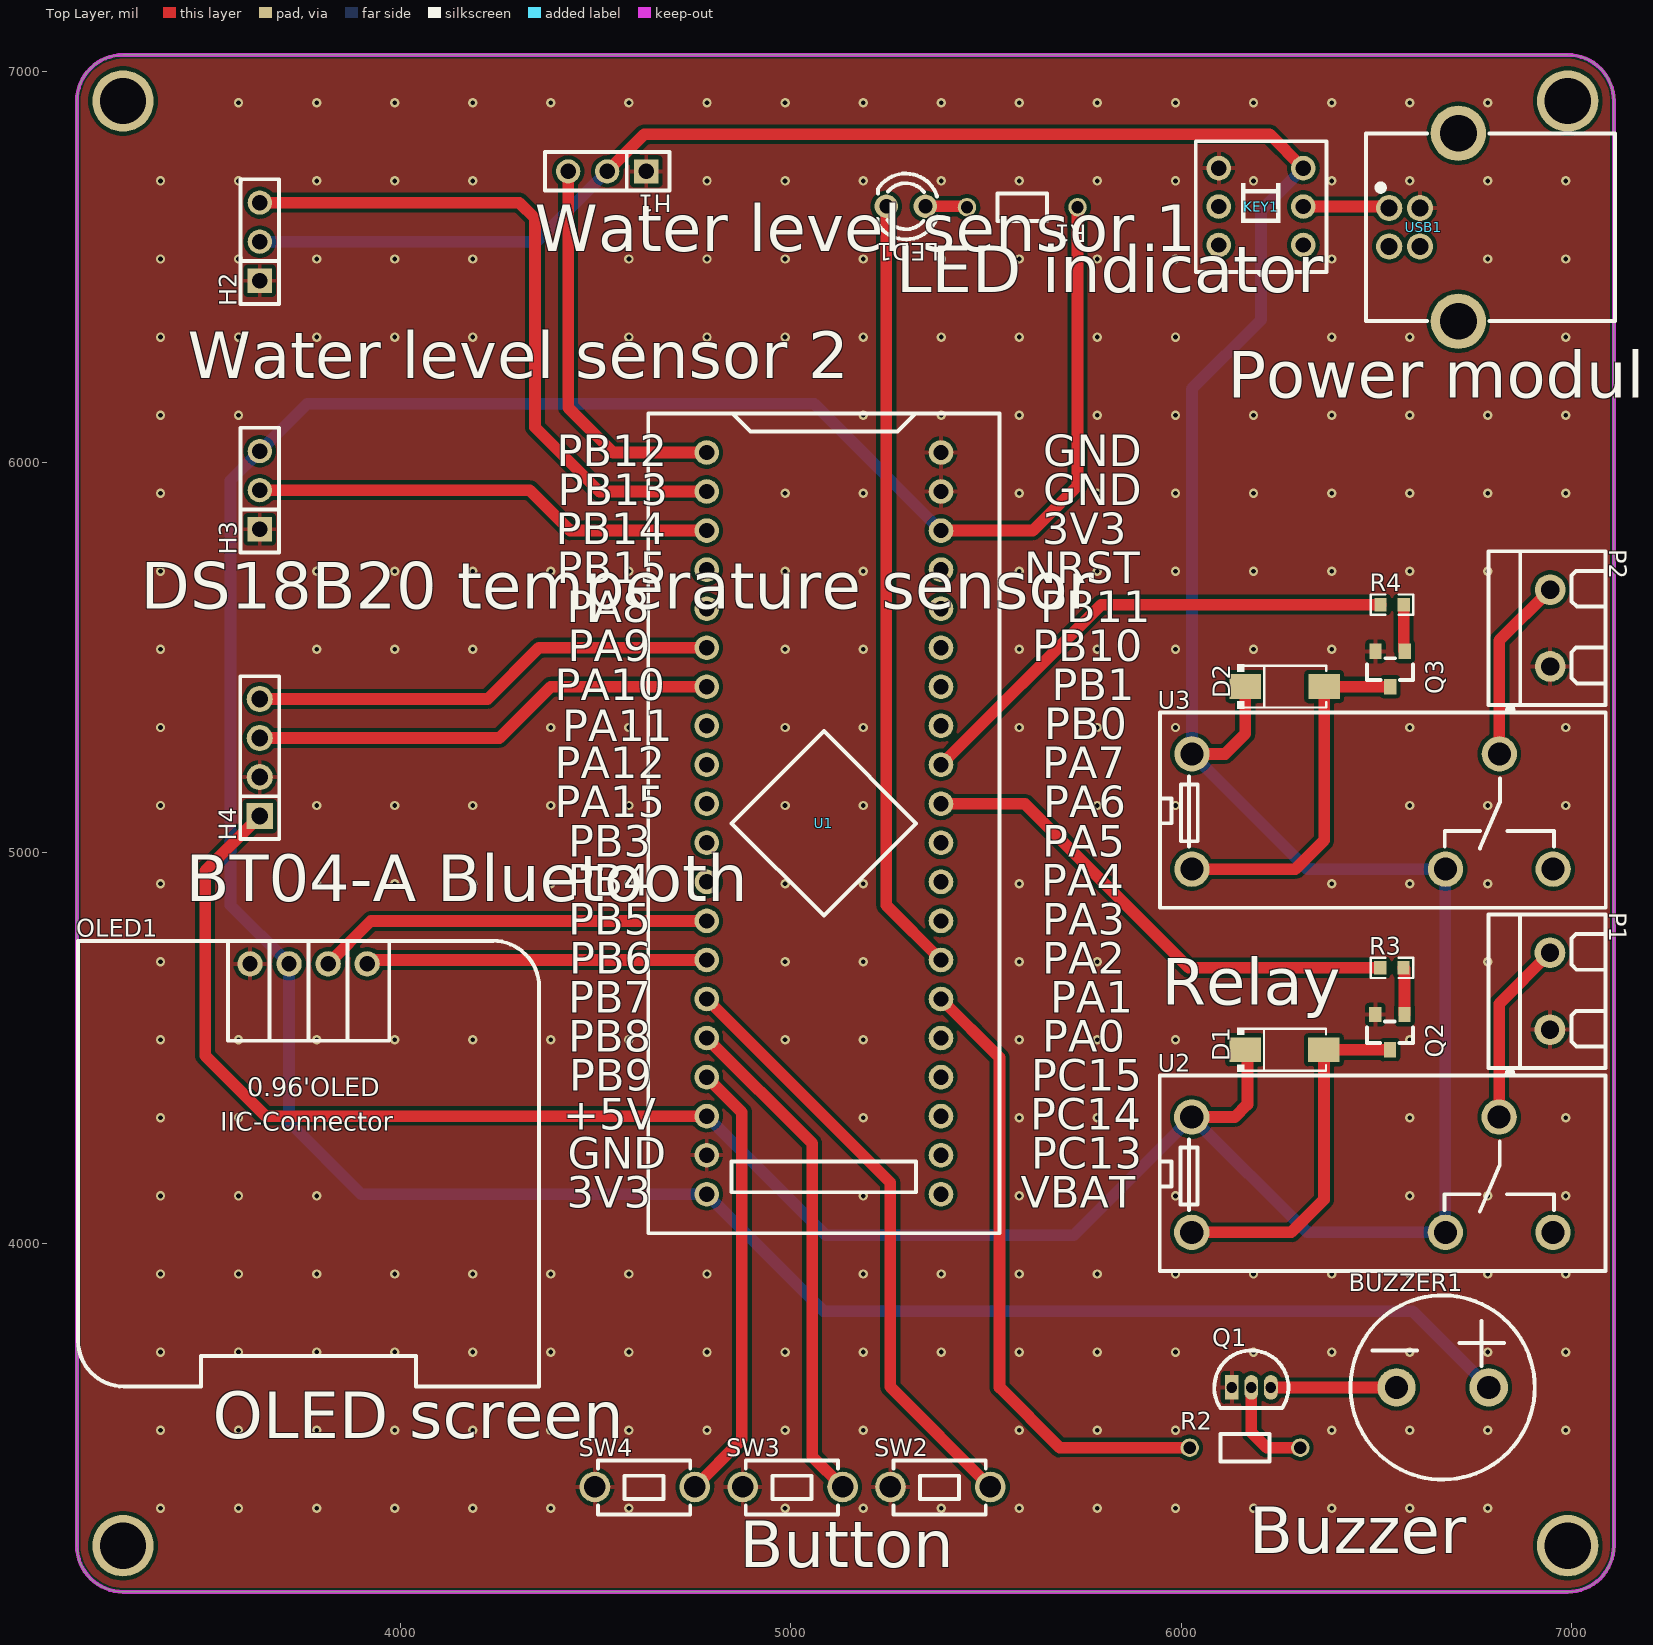
[diagram p0: Top Layer view]
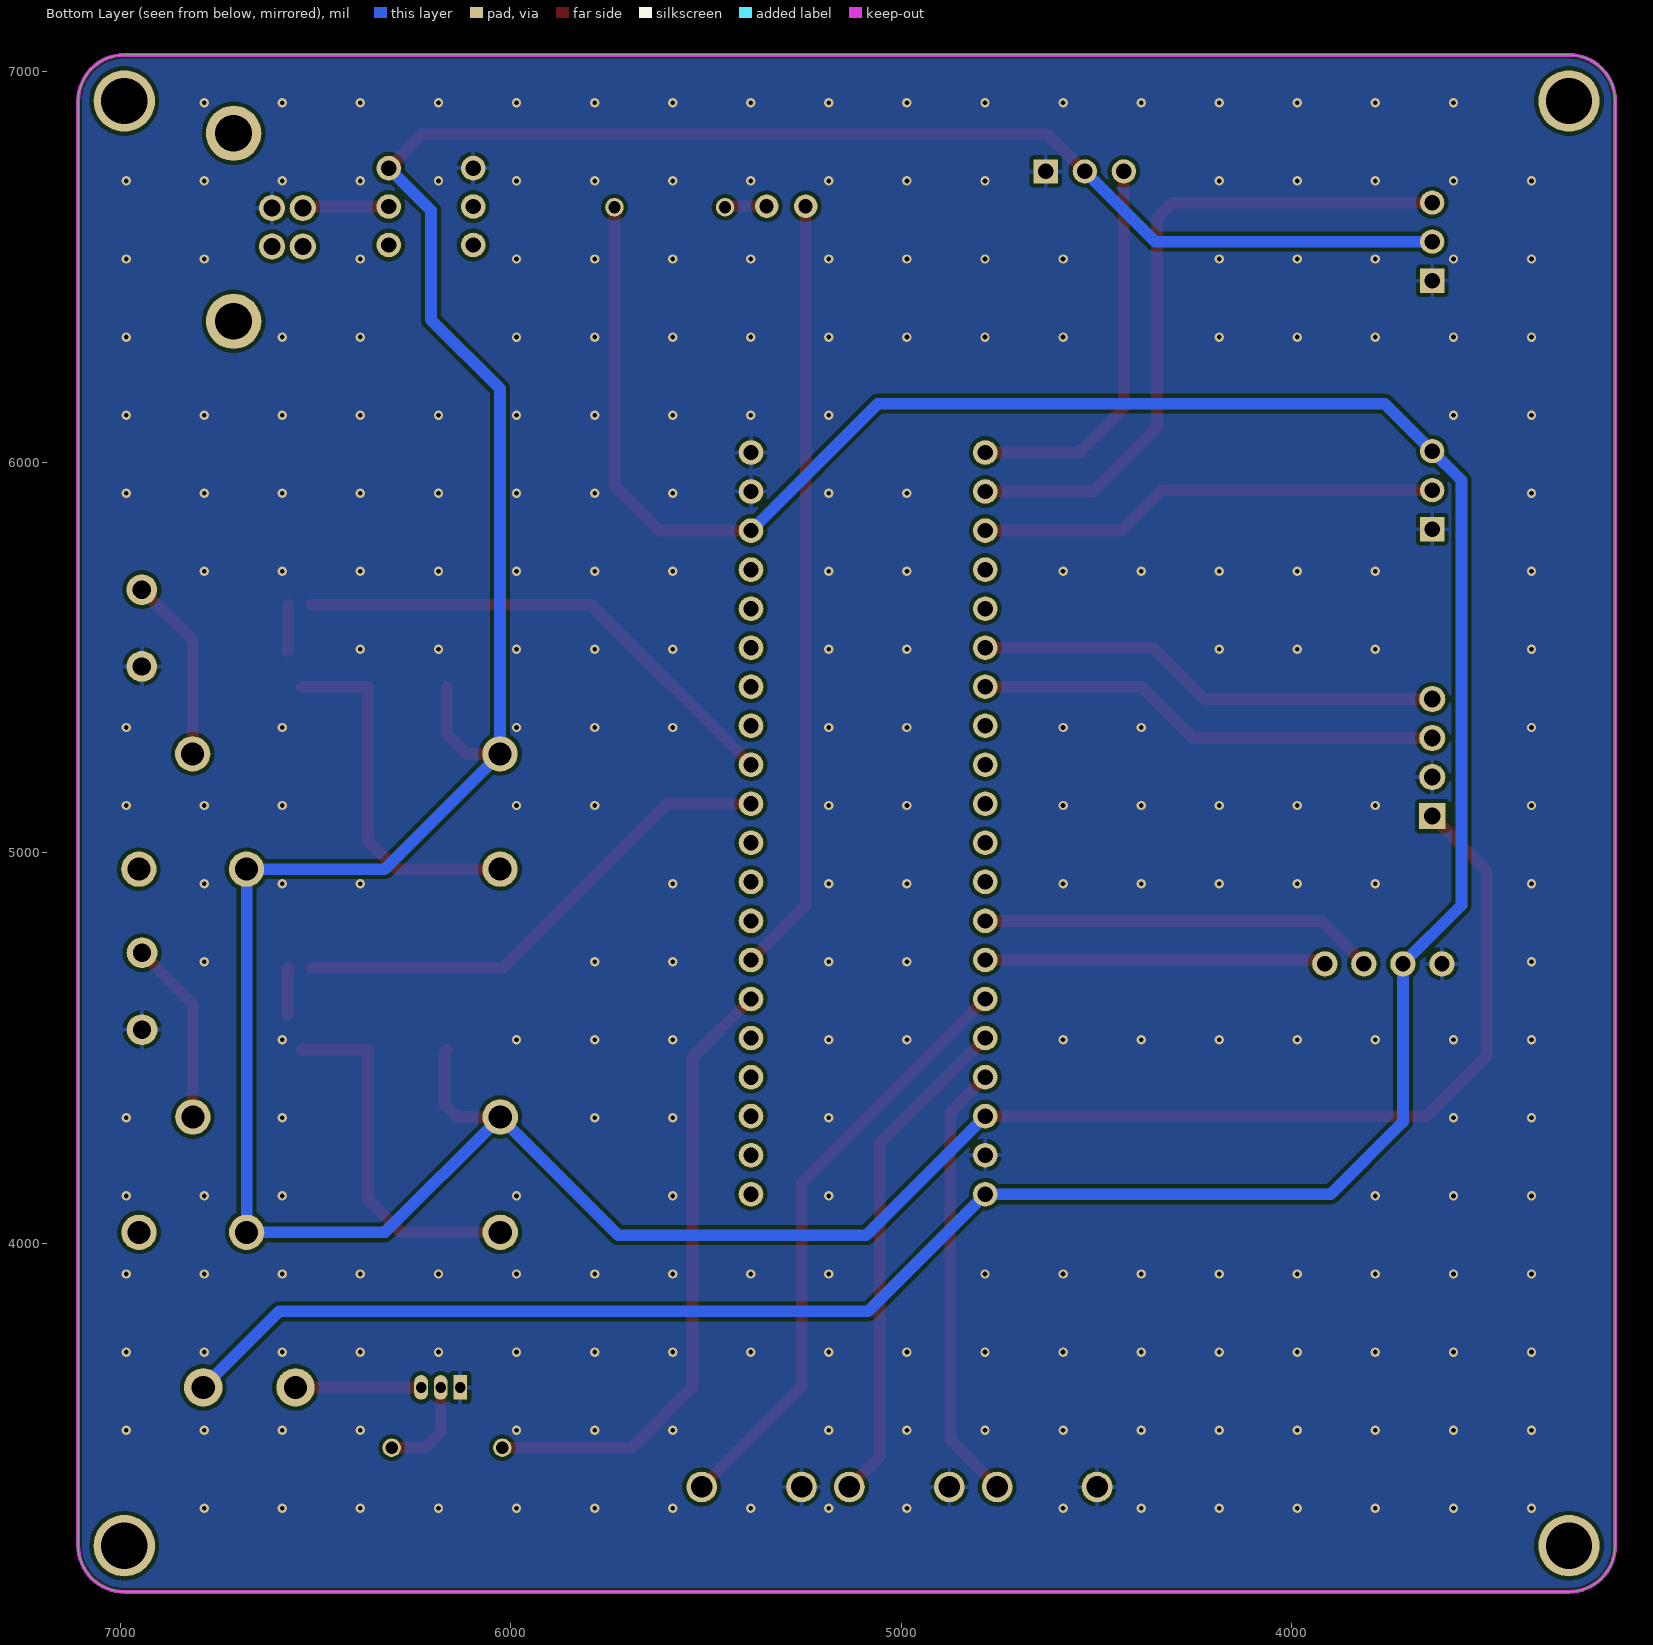
[diagram p1: Bottom Layer view, seen from below]
# Altium PCB MISC89014.pcbdoc
Units mil, origin at the board's own origin, x right, y up, seen from the top; angles counter-clockwise.
Board outline 3937.01 x 3937.01 mil, 2 copper layers (Top Layer, Bottom Layer), stack 62.206 mil thick; 26 components, 47 nets, 118 pads, 256 vias.

## Layer stack, top to bottom
Top Solder Mask Layer: solder mask 0.394, Dk 3.3
Top Layer: signal copper 1.379
Dielectric1: surface 59.449, FR4, Dk 4.5
Bottom Layer: signal copper 1.378
Bottom Solder Mask Layer: solder mask 0.394, Dk 3.3

## Board outline
6990.39,3106.5 ccw(c6990.39,3224.61) 7108.5,3224.61 7108.5,6925.39 ccw(c6990.39,6925.39) 6990.39,7043.5 3289.61,7043.5 ccw(c3289.61,6925.39) 3171.5,6925.39 3171.5,3224.61 ccw(c3289.61,3224.61) 3289.61,3106.5

## Design rules (kind name [scope] priority, off if disabled: settings)
BoardOutlineClearance copperThickness2oz_1 [All] p2 off: genericclearance=7.99 ignorepadtopadclearanceinfootprint=FALSE except(0: Arc-SplitContinuation Track-SplitContinuation SMDPad-SplitContinuation THPad-SplitContinuation Via-SplitContinuation Fill-SplitContinuation Region-SplitContinuation Poly-SplitContinuation Text-SplitContinuation Hole-SplitContinuation; 5.98: Arc-CutoutEdge Track-CutoutEdge SMDPad-CutoutEdge THPad-CutoutEdge Via-CutoutEdge Text-CutoutEdge; 6.89: Hole-OutlineEdge Hole-CutoutEdge; 10: Poly-OutlineEdge Poly-CutoutEdge; 11.81: Arc-OutlineEdge Track-OutlineEdge SMDPad-OutlineEdge THPad-OutlineEdge Via-OutlineEdge Fill-OutlineEdge Region-OutlineEdge Text-OutlineEdge Fill-CutoutEdge Region-CutoutEdge)
BoardOutlineClearance Plane_innerPlane_1 [All] p4 off: genericclearance=4.02 ignorepadtopadclearanceinfootprint=FALSE except(0: Arc-SplitContinuation Track-SplitContinuation SMDPad-SplitContinuation THPad-SplitContinuation Via-SplitContinuation Fill-SplitContinuation Region-SplitContinuation Poly-SplitContinuation Text-SplitContinuation Hole-SplitContinuation; 5.98: Arc-CutoutEdge Track-CutoutEdge SMDPad-CutoutEdge THPad-CutoutEdge Via-CutoutEdge Text-CutoutEdge; 6.89: Hole-OutlineEdge Hole-CutoutEdge; 10: Poly-OutlineEdge Poly-CutoutEdge; 11.81: Arc-OutlineEdge Track-OutlineEdge SMDPad-OutlineEdge THPad-OutlineEdge Via-OutlineEdge Fill-OutlineEdge Region-OutlineEdge Text-OutlineEdge Fill-CutoutEdge Region-CutoutEdge)
BoardOutlineClearance Copper_copperRegion_1 [All] p6 off: genericclearance=4.02 ignorepadtopadclearanceinfootprint=FALSE except(0: Arc-SplitContinuation Track-SplitContinuation SMDPad-SplitContinuation THPad-SplitContinuation Via-SplitContinuation Fill-SplitContinuation Region-SplitContinuation Poly-SplitContinuation Text-SplitContinuation Hole-SplitContinuation; 5.98: Arc-CutoutEdge Track-CutoutEdge SMDPad-CutoutEdge THPad-CutoutEdge Via-CutoutEdge Text-CutoutEdge; 6.89: Hole-OutlineEdge Hole-CutoutEdge; 10: Poly-OutlineEdge Poly-CutoutEdge; 11.81: Arc-OutlineEdge Track-OutlineEdge SMDPad-OutlineEdge THPad-OutlineEdge Via-OutlineEdge Fill-OutlineEdge Region-OutlineEdge Text-OutlineEdge Fill-CutoutEdge Region-CutoutEdge)
BoardOutlineClearance copperThickness1oz_1 [All] p8: genericclearance=4.02 ignorepadtopadclearanceinfootprint=FALSE except(0: Arc-SplitContinuation Track-SplitContinuation SMDPad-SplitContinuation THPad-SplitContinuation Via-SplitContinuation Fill-SplitContinuation Region-SplitContinuation Poly-SplitContinuation Text-SplitContinuation Hole-SplitContinuation; 5.98: Arc-CutoutEdge Track-CutoutEdge SMDPad-CutoutEdge THPad-CutoutEdge Via-CutoutEdge Text-CutoutEdge; 6.89: Hole-OutlineEdge Hole-CutoutEdge; 10: Poly-OutlineEdge Poly-CutoutEdge; 11.81: Arc-OutlineEdge Track-OutlineEdge SMDPad-OutlineEdge THPad-OutlineEdge Via-OutlineEdge Fill-OutlineEdge Region-OutlineEdge Text-OutlineEdge Fill-CutoutEdge Region-CutoutEdge)
Clearance copperThickness2oz [All] p1 off: gap=7.99 ignorepadtopadclearanceinfootprint=FALSE except(5.98: SMDPad-Track SMDPad-SMDPad THPad-Track SMDPad-THPad THPad-THPad Track-Via SMDPad-Via THPad-Via Via-Via Fill-SMDPad Region-SMDPad Fill-THPad Region-THPad Fill-Via Region-Via Fill-Fill Fill-Region Region-Region Arc-Track Arc-SMDPad Arc-THPad Arc-Via Fill-Arc Region-Arc Arc-Arc Text-Track SMDPad-Text Text-THPad Text-Via Fill-Text Region-Text Arc-Text Text-Text; 6.89: Hole-Track Hole-SMDPad Hole-THPad Hole-Via Fill-Hole Region-Hole Hole-Arc Hole-Text; 10: Poly-Track Poly-SMDPad Poly-THPad Poly-Via Poly-Fill Poly-Region Poly-Poly Poly-Arc Poly-Text Poly-Hole; 11.81: Fill-Track Region-Track)
Clearance Plane_innerPlane [All] p3 off: gap=4.02 ignorepadtopadclearanceinfootprint=FALSE except(5.98: SMDPad-Track SMDPad-SMDPad THPad-Track SMDPad-THPad THPad-THPad Track-Via SMDPad-Via THPad-Via Via-Via Fill-SMDPad Region-SMDPad Fill-THPad Region-THPad Fill-Via Region-Via Fill-Fill Fill-Region Region-Region Arc-Track Arc-SMDPad Arc-THPad Arc-Via Fill-Arc Region-Arc Arc-Arc Text-Track SMDPad-Text Text-THPad Text-Via Fill-Text Region-Text Arc-Text Text-Text; 6.89: Hole-Track Hole-SMDPad Hole-THPad Hole-Via Fill-Hole Region-Hole Hole-Arc Hole-Text; 10: Poly-Track Poly-SMDPad Poly-THPad Poly-Via Poly-Fill Poly-Region Poly-Poly Poly-Arc Poly-Text Poly-Hole; 11.81: Fill-Track Region-Track)
Clearance Copper_copperRegion [All] p5 off: gap=4.02 ignorepadtopadclearanceinfootprint=FALSE except(5.98: SMDPad-Track SMDPad-SMDPad THPad-Track SMDPad-THPad THPad-THPad Track-Via SMDPad-Via THPad-Via Via-Via Fill-SMDPad Region-SMDPad Fill-THPad Region-THPad Fill-Via Region-Via Fill-Fill Fill-Region Region-Region Arc-Track Arc-SMDPad Arc-THPad Arc-Via Fill-Arc Region-Arc Arc-Arc Text-Track SMDPad-Text Text-THPad Text-Via Fill-Text Region-Text Arc-Text Text-Text; 6.89: Hole-Track Hole-SMDPad Hole-THPad Hole-Via Fill-Hole Region-Hole Hole-Arc Hole-Text; 10: Poly-Track Poly-SMDPad Poly-THPad Poly-Via Poly-Fill Poly-Region Poly-Poly Poly-Arc Poly-Text Poly-Hole; 11.81: Fill-Track Region-Track)
Clearance copperThickness1oz [All] p7: gap=4.02 ignorepadtopadclearanceinfootprint=FALSE except(5.98: SMDPad-Track SMDPad-SMDPad THPad-Track SMDPad-THPad THPad-THPad Track-Via SMDPad-Via THPad-Via Via-Via Fill-SMDPad Region-SMDPad Fill-THPad Region-THPad Fill-Via Region-Via Fill-Fill Fill-Region Region-Region Arc-Track Arc-SMDPad Arc-THPad Arc-Via Fill-Arc Region-Arc Arc-Arc Text-Track SMDPad-Text Text-THPad Text-Via Fill-Text Region-Text Arc-Text Text-Text; 6.89: Hole-Track Hole-SMDPad Hole-THPad Hole-Via Fill-Hole Region-Hole Hole-Arc Hole-Text; 10: Poly-Track Poly-SMDPad Poly-THPad Poly-Via Poly-Fill Poly-Region Poly-Poly Poly-Arc Poly-Text Poly-Hole; 11.81: Fill-Track Region-Track)
DiffPairsRouting differentialPair [All] p1: maxlimit=6 minlimit=6 mostfreqgap=6 toplayer_minwidth=5 toplayer_prefwidth=10 toplayer_maxwidth=100 toplayer_mingap=6 toplayer_prefgap=6 toplayer_maxgap=6 bottomlayer_minwidth=5 bottomlayer_prefwidth=10 bottomlayer_maxwidth=100 bottomlayer_mingap=6 bottomlayer_prefgap=6 bottomlayer_maxgap=6 maxuncoupledlength=10
HoleToHoleClearance otherClearance [All] p1: gap=11.81 allowstackedmicrovias=TRUE
Length netLength [All] p1: minlimit=0 maxlimit=0
PasteMaskExpansion pasteMaskExpansion [All] p1: expansion=0
PlaneConnect innerPlane [All] p1: planeconnectstyle=Relief reliefexpansion=20 reliefentries=4 reliefconductorwidth=10 reliefairgap=10
PolygonConnect copperRegion [All] p1: connectstyle=Relief reliefconductorwidth=10 reliefentries=4 polygonreliefangle="90 Angle" airgapwidth=10 via.connectstyle=Relief via.reliefconductorwidth=10 via.reliefentries=4 via.polygonreliefangle="90 Angle" via.airgapwidth=10
RoutingVias viaSize [All] p1: holewidth=12.01 width=24.02 viastyle="Through Hole" minholewidth=11.81 minwidth=19.68 maxholewidth=248.03 maxwidth=393.7
SolderMaskExpansion solderMaskExpansion [IsVia] p1: expansion=-1000 istentingtop=TRUE
SolderMaskExpansion solderMaskExpansion [All] p2: expansion=2.01 istentingtop=FALSE
Width copperThickness2oz_2 [All] p1 off: maxlimit=100 minlimit=8 preferedwidth=10
Width copperThickness1oz_2 [All] p2: maxlimit=100 minlimit=5 preferedwidth=30

## Components (designator, comment, footprint, x,y, rotation, side; value= is the part's Value field where it differs from the comment)
BUZZER1 "buzzer" BUZ-TH_BD12.0-P6.00-D0.9-RD 6670,3630 r0 top
D1 "" SMA_1N4007 6265,4495 r0 top
D2 "" SMA_1N4007 6265.47,5425.24 r0 top
H1 "" HDR-TH_3P-P2.54-V-F 4530,6745 r180 top
H2 "" HDR-TH_3P-P2.54-V-F 3640,6565 r90 top
H3 "" HDR-TH_3P-P2.54-V-F 3640,5928.44 r90 top
H4 "" HDR-TH_4P-P2.54-V-F 3640,5243.46 r90 top
KEY1 "Non-self-locking switch 8.5×8.5 silent" SW-TH_6P-L8.5-W8.5-P2.54 6205,6655 r90 top
LED1 "" LED_TH-3mm 5294.9,6655.74 r180 top
OLED1 "" 0.96OLED_4P 3765,4715 r0 top
P1 "KF301-2P terminal block" CONN-TH_XY301V-A-5.0-2P 6945,4645 r270 top
P2 "KF301-2P terminal block" CONN-TH_XY301V-A-5.0-2P 6945.47,5575.24 r270 top
Q1 "" S8050_TO_92 6180,3630 r0 top
Q2 "" S8050_SOT-23 6535,4540 r90 top
Q3 "" S8050_SOT-23 6535.47,5470.24 r90 top
R1 "220" Res_1/8W 5593.23,6655.74 r180 top
R2 "10kΩ" Res_1/8W 6163.81,3473.19 r0 top
R3 "1K" R0603 6540,4705 r0 top
R4 "1K" R0603 6540.47,5635.24 r0 top
SW2 "" Key_TH_3.5x6x4.3 5377.07,3375 r0 top
SW3 "" Key_TH_3.5x6x4.3 4998.53,3375 r0 top
SW4 "" Key_TH_3.5x6x4.3 4620,3375 r0 top
U1 "STM32F103C8T6-Card" CONN-TH_L53.3-W22.9_STM32F103C8T6-CARD 5085,5075 r270 top
U2 "SSKD6132" RELAY-TH_G2R-1 6490,4175 r0 top
U3 "SSKD6132" RELAY-TH_G2R-1 6490.47,5105.24 r0 top
USB1 "" "USB_ Type-B" 6790.29,6596.4 r90 top

## Footprints (in the part's own frame and the unit in brackets; to place one, negate y for a bottom-side part, rotate by r counter-clockwise, add the part's x,y. Pads: shape width x height; smd on the part's side, far side on the other; paste and mask are expansions set on the pad)
0.96OLED_4P [mm]
  round 1.65 hole 1 copper offset 0,0: 1(-3.81,-0.001) 2(-1.27,0.002) 3(1.27,0.002) 4(3.81,0.002)
  silkscreen extent -15,-27.5 15,1.5
BUZ-TH_BD12.0-P6.00-D0.9-RD [mm]
  round 2.5 hole 1.5 paste+0 mask+0.05: 1(-3,0) 2(3,0)
  silkscreen extent -5.99,-5.99 5.99,5.99
CONN-TH_L53.3-W22.9_STM32F103C8T6-CARD [mm]
  round 1.6 hole 1: 1(-24.13,-7.62) 2(-21.59,-7.62) 3(-19.05,-7.62) 4(-16.51,-7.62) 5(-13.97,-7.62) 6(-11.43,-7.62) 7(-8.89,-7.62) 8(-6.35,-7.62) 9(-3.81,-7.62) 10(-1.27,-7.62) 11(1.27,-7.62) 12(3.81,-7.62) 13(6.35,-7.62) 14(8.89,-7.62) 15(11.43,-7.62) 16(13.97,-7.62) 17(16.51,-7.62) 18(19.05,-7.62) 19(21.59,-7.62) 20(24.13,-7.62) 21(24.13,7.62) 22(21.59,7.62) 23(19.05,7.62) 24(16.51,7.62) 25(13.97,7.62) 26(11.43,7.62) 27(8.89,7.62) 28(6.35,7.62) 29(3.81,7.62) 30(1.27,7.62) 31(-1.27,7.62) 32(-3.81,7.62) 33(-6.35,7.62) 34(-8.89,7.62) 35(-11.43,7.62) 36(-13.97,7.62) 37(-16.51,7.62) 38(-19.05,7.62) 39(-21.59,7.62) 40(-24.13,7.62)
  silkscreen extent -26.67,-11.43 26.67,11.43
CONN-TH_XY301V-A-5.0-2P [mm]
  round 2 hole 1.2: 1(-2.5,0) 2(2.5,0)
  silkscreen extent -5,-4 5.6,3.6
HDR-TH_3P-P2.54-V-F [mil]
  rect 62x62 hole 40.16: 1(-100,0)
  round 62 hole 40.16: 2(0,0) 3(100,0)
  silkscreen extent -160,-49 160,49
HDR-TH_4P-P2.54-V-F [mm]
  rect 1.7x1.7 hole 1.1: 1(-3.81,0)
  round 1.7 hole 1.1: 2(-1.27,0) 3(1.27,0) 4(3.81,0)
  silkscreen extent -5.29,-1.27 5.29,1.27
Key_TH_3.5x6x4.3 [mil]
  round 78.7 hole 55.1 paste+0 mask+2: A(-121.44,0) B(134.46,0)
  silkscreen extent -114,-70 123,68
LED_TH-3mm [mil]
  round 60 hole 36 paste+0 mask+2: 1(-50,0) 2(50,0)
  silkscreen extent -81,-84 72,85
R0603 [mil]
  rect 31.75x34.02 smd paste-3937.01 mask+2: 1(-29.66,0) 2(29.66,0)
  silkscreen extent -55,-26 55,26
RELAY-TH_G2R-1 [mm]
  round 2.3 hole 1.5: 1(-11.75,-3.75) 2(4.75,-3.75) 3(11.75,-3.75) 4(8.25,3.75) 5(-11.75,3.75)
  silkscreen extent -13.83,-6.26 15.17,6.44
Res_1/8W [mil]
  round 47.2 hole 31.5 paste+0 mask+2: 1(-141.7,2.48) 2(141.7,2.48)
  silkscreen extent -63,-33 63,38
S8050_SOT-23 [mm]
  rect 1x0.8 smd paste+0 mask+0.051: 1(1.15,-0.95) 2(1.15,0.95) 3(-1.15,0)
  silkscreen extent -0.7,-1.5 0.7,1.5
S8050_TO_92 [mil]
  rect 35.4x63 hole 27.6 paste+0 mask+2: 1(-50,0)
  oval 35.4x63 hole 27.6 paste+0 mask+2: 2(0,0) 3(50,0)
  silkscreen extent -95,-53 95,95
SMA_1N4007 [mil]
  rect 80.57x63.78 smd paste+0 mask+2: 1(-101,0) 2(101,0)
  silkscreen extent -121,-57 106,57
SW-TH_6P-L8.5-W8.5-P2.54 [mm]
  round 1.6 hole 1: 1(-2.5,-2.75) 2(0,-2.75) 3(2.5,-2.75) 4(-2.5,2.75) 5(0,2.75) 6(2.5,2.75)
  silkscreen extent -4.47,-4.25 4.25,4.25
"USB_ Type-B" [mm]
  round 1.7 hole 1.1 copper offset 0,0 paste+0 mask+0.051: 1(1.39,6.532) 2(-1.11,6.532) 3(-1.11,4.532) 4(1.39,4.532)
  round 3.6 hole 2.4 paste+0 mask+0.051: 5(-5.977,2.032) 5(6.256,2.032)
  silkscreen extent -5.96,-8.17 6.25,8.03

## Free pads (board coordinates)
  round 157.48 hole 118.11: 1(3289.61,6925.39) 1(3289.61,3224.61) 1(6990.39,6925.39) 1(6990.39,3224.61)

## Via types
v1: diameter 24.02, hole 12, Top Layer to Bottom Layer, 256 vias

## Nets (pads, with @x,y where several pads share a name; then routed paths per layer and width w, separated by ;. In a path a pad name is that pad's centre, name@x,y a point inside that pad or via, vN(x,y) a via of type N, cw(c..) or ccw(c..) an arc to the next point about the centre after c; other vN are vias at no path point)
$1N18282: KEY1.2 USB1.1 | length 221.5
  Top Layer w30: KEY1.2 6529.25,6654.99 USB1.1
$1N18294: LED1.1 R1.2 | length 107.7
  Top Layer w30: LED1.1 5449.05,6655.74 R1.2
$1N18316: BUZZER1.1 Q1.3 | length 321.9
  Top Layer w30: Q1.3 BUZZER1.1
$1N18319: Q1.2 R2.2 | length 256.8
  Top Layer w30: Q1.2 6180,3515 6219.34,3475.66 R2.2
$1N18331: D1.2 Q2.3 U2.1 | length 926.4
  Top Layer w30: U2.1 6282.35,4027.35 6366,4111 D1.2 6534.72,4495 Q2.3
$1N18332: Q2.1 R3.2 | length 120.9
  Top Layer w30: R3.2 6572.4,4702.26 Q2.1
$1N18336: P1.1 U2.4 | length 474.7
  Top Layer w30: U2.4 6814.8,4613.23 P1.1
$1N18339: P2.1 U3.4 | length 474.7
  Top Layer w30: U3.4 6815.27,5543.47 P2.1
$1N18343: Q3.1 R4.2 | length 120.9
  Top Layer w30: R4.2 6570.13,5518.26 Q3.1
$1N18344: D2.2 Q3.3 U3.1 | length 932.1
  Top Layer w30: U3.1 6292.59,4957.59 6366.47,5031.47 D2.2 6535.19,5425.24 Q3.3
+5V: D1.1 D2.1 H1.2 H2.2 H4.1 KEY1.3 U1.18 U2.2 U2.5 U3.2 U3.5 | length 11008
  Top Layer w30: H4.1 3500,4953.46 3500,4480 3655,4325 U1.18 ; H1.2 4625,6840 6226.69,6840 KEY1.3 ; U2.5 6137.65,4322.65 6170,4355 6170,4489 D1.1 ; U3.5 6112.89,5252.89 6164.47,5304.47 D2.1
  Bottom Layer w30: H2.2 4350,6565 H1.2 ; U1.18 5090,4020 5724.75,4020 U2.5 6322.7,4027.35 U2.2 6677,4957.12 U3.2 6323.17,4957.59 U3.5 6027.87,6187.87 6205,6365 6205,6645.15 KEY1.3
GND: H1.1 H2.1 H3.1 H4.2 KEY1.6 OLED1.1 P1.2 P2.2 Q1.1 Q2.2 Q3.2 SW2.A SW3.A SW4.A U1.19 U1.39 U1.40 USB1.4
  other v1: 3385.6,3320.6 3585.6,3320.6 3785.6,3320.6 3985.6,3320.6 4185.6,3320.6 4385.6,3320.6 4585.6,3320.6 4985.6,3320.6 5185.6,3320.6 5385.6,3320.6 5585.6,3320.6 5785.6,3320.6 5985.6,3320.6 6185.6,3320.6 6385.6,3320.6 6585.6,3320.6 6785.6,3320.6 3385.6,3520.6 3585.6,3520.6 3785.6,3520.6 3985.6,3520.6 4185.6,3520.6 4385.6,3520.6 4585.6,3520.6 4785.6,3520.6 4985.6,3520.6 5185.6,3520.6 5585.6,3520.6 5785.6,3520.6 5985.6,3520.6 6385.6,3520.6 6585.6,3520.6 6785.6,3520.6 6985.6,3520.6 3385.6,3720.6 3585.6,3720.6 3785.6,3720.6 3985.6,3720.6 4185.6,3720.6 4385.6,3720.6 4585.6,3720.6 4785.6,3720.6 4985.6,3720.6 5185.6,3720.6 5385.6,3720.6 5585.6,3720.6 5785.6,3720.6 5985.6,3720.6 6185.6,3720.6 6385.6,3720.6 6585.6,3720.6 6785.6,3720.6 6985.6,3720.6 3385.6,3920.6 3585.6,3920.6 3785.6,3920.6 3985.6,3920.6 4185.6,3920.6 4385.6,3920.6 4585.6,3920.6 4785.6,3920.6 5185.6,3920.6 5385.6,3920.6 5585.6,3920.6 5785.6,3920.6 5985.6,3920.6 6185.6,3920.6 6385.6,3920.6 6585.6,3920.6 6785.6,3920.6 6985.6,3920.6 3385.6,4120.6 3585.6,4120.6 3785.6,4120.6 5185.6,4120.6 5585.6,4120.6 5985.6,4120.6 6585.6,4120.6 6785.6,4120.6 6985.6,4120.6 3385.6,4320.6 3585.6,4320.6 5185.6,4320.6 5585.6,4320.6 5785.6,4320.6 6585.6,4320.6 6985.6,4320.6 3385.6,4520.6 3585.6,4520.6 3785.6,4520.6 3985.6,4520.6 4185.6,4520.6 4385.6,4520.6 4585.6,4520.6 4985.6,4520.6 5185.6,4520.6 5585.6,4520.6 5785.6,4520.6 5985.6,4520.6 6585.6,4520.6 3385.6,4720.6 4985.6,4720.6 5185.6,4720.6 5585.6,4720.6 5785.6,4720.6 6785.6,4720.6 3385.6,4920.6 3785.6,4920.6 3985.6,4920.6 4185.6,4920.6 4385.6,4920.6 4585.6,4920.6 4985.6,4920.6 5185.6,4920.6 5585.6,4920.6 6385.6,4920.6 6585.6,4920.6 6785.6,4920.6 3385.6,5120.6 3785.6,5120.6 3985.6,5120.6 4185.6,5120.6 4385.6,5120.6 4585.6,5120.6 4985.6,5120.6 5185.6,5120.6 5785.6,5120.6 5985.6,5120.6 6585.6,5120.6 6785.6,5120.6 6985.6,5120.6 3385.6,5320.6 4385.6,5320.6 4585.6,5320.6 4985.6,5320.6 5185.6,5320.6 5585.6,5320.6 5785.6,5320.6 5985.6,5320.6 6585.6,5320.6 6985.6,5320.6 3385.6,5520.6 3785.6,5520.6 3985.6,5520.6 4185.6,5520.6 4985.6,5520.6 5185.6,5520.6 5585.6,5520.6 5785.6,5520.6 5985.6,5520.6 6185.6,5520.6 6385.6,5520.6 3385.6,5720.6 3785.6,5720.6 3985.6,5720.6 4185.6,5720.6 4385.6,5720.6 4585.6,5720.6 4985.6,5720.6 5185.6,5720.6 5585.6,5720.6 5785.6,5720.6 5985.6,5720.6 6185.6,5720.6 6385.6,5720.6 6585.6,5720.6 6785.6,5720.6 3385.6,5920.6 4985.6,5920.6 5185.6,5920.6 5585.6,5920.6 5785.6,5920.6 5985.6,5920.6 6185.6,5920.6 6385.6,5920.6 6585.6,5920.6 6785.6,5920.6 6985.6,5920.6 3385.6,6120.6 3585.6,6120.6 5185.6,6120.6 5385.6,6120.6 5585.6,6120.6 5785.6,6120.6 5985.6,6120.6 6185.6,6120.6 6385.6,6120.6 6585.6,6120.6 6785.6,6120.6 6985.6,6120.6 3385.6,6320.6 3585.6,6320.6 3785.6,6320.6 3985.6,6320.6 4185.6,6320.6 4585.6,6320.6 4785.6,6320.6 4985.6,6320.6 5185.6,6320.6 5385.6,6320.6 5585.6,6320.6 5785.6,6320.6 5985.6,6320.6 6385.6,6320.6 6585.6,6320.6 6985.6,6320.6 3385.6,6520.6 3585.6,6520.6 3785.6,6520.6 3985.6,6520.6 4185.6,6520.6 4585.6,6520.6 4785.6,6520.6 4985.6,6520.6 5185.6,6520.6 5385.6,6520.6 5585.6,6520.6 5785.6,6520.6 5985.6,6520.6 6385.6,6520.6 6785.6,6520.6 6985.6,6520.6 3385.6,6720.6 3585.6,6720.6 3785.6,6720.6 3985.6,6720.6 4185.6,6720.6 4785.6,6720.6 4985.6,6720.6 5185.6,6720.6 5385.6,6720.6 5585.6,6720.6 5785.6,6720.6 5985.6,6720.6 6185.6,6720.6 6385.6,6720.6 6585.6,6720.6 6785.6,6720.6 6985.6,6720.6 3585.6,6920.6 3785.6,6920.6 3985.6,6920.6 4185.6,6920.6 4385.6,6920.6 4585.6,6920.6 4785.6,6920.6 4985.6,6920.6 5185.6,6920.6 5385.6,6920.6 5585.6,6920.6 5785.6,6920.6 5985.6,6920.6 6185.6,6920.6 6385.6,6920.6 6585.6,6920.6 6785.6,6920.6
NRST: U1.37
PA0: U1.25
PA1: R2.1 U1.26 | length 1608.2
  Top Layer w30: U1.26 5535,4475 5535,3630 5689.34,3475.66 R2.1
PA2: LED1.2 U1.27 | length 1988.8
  Top Layer w30: LED1.2 5244.9,4865.1 U1.27
PA3: U1.28
PA4: U1.29
PA5: U1.30
PA6: R3.1 U1.31 | length 1299.3
  Top Layer w30: U1.31 5600,5125 6020,4705 R3.1
PA7: R4.1 U1.32 | length 1295.7
  Top Layer w30: U1.32 5795.25,5635.24 R4.1
PA8: U1.5
PA9: H4.4 U1.6 | length 1199.5
  Top Layer w30: H4.4 4223.46,5393.46 4355,5525 U1.6
PA10: H4.3 U1.7 | length 1199.5
  Top Layer w30: H4.3 4253.46,5293.46 4385,5425 U1.7
PA11: U1.8
PA12: U1.9
PA15: U1.10
PB0: U1.33
PB1: U1.34
PB3: U1.11
PB4: U1.12
PB5: OLED1.3 U1.13 | length 1015.5
  Top Layer w30: OLED1.3@3815,4715.05 3924.95,4825 U1.13
PB6: OLED1.4 U1.14 | length 874.1
  Top Layer w30: OLED1.4@3915,4715.05 3924.95,4725 U1.14
PB7: SW2.B U1.15 | length 1550.9
  Top Layer w30: U1.15 5255,4155 5255,3631.53 SW2.B
PB8: SW3.B U1.16 | length 1294.1
  Top Layer w30: U1.16 5055,4255 5055,3452.99 SW3.B
PB9: SW4.B U1.17 | length 1137.2
  Top Layer w30: SW4.B 4875,3495.54 4875,4335 U1.17
PB10: U1.35
PB11: U1.36
PB12: H1.3 U1.1 | length 1007.6
  Top Layer w30: H1.3 4430,6140 4545,6025 U1.1
PB13: H2.3 U1.2 | length 1764.9
  Top Layer w30: H2.3 4305,6665 4345,6625 4345,6090 4510,5925 U1.2
PB14: H3.2 U1.3 | length 1187.8
  Top Layer w30: H3.2 4331.56,5928.44 4435,5825 U1.3
PB15: U1.4
PC13: U1.22
PC14: U1.23
PC15: U1.24
VBAT: U1.21
VCC: BUZZER1.2 H3.3 OLED1.2 R1.1 U1.20 U1.38 | length 8207.3
  Top Layer w30: U1.38 5620,5825 5734.93,5939.93 R1.1
  Bottom Layer w30: U1.38 5060,6150 3761.56,6150 H3.3 3565,5953.44 3565,4865.05 3715,4715.05 3715,4310 3900,4125 U1.20 5085,3825 6593.11,3825 BUZZER1.2
pads on no net: KEY1.1 KEY1.4 KEY1.5 U2.3 U3.3 USB1.2 USB1.3 USB1.5

## Polygon pours and split planes (outlines as drawn)
GND on Bottom Layer (solid, remove dead copper, pour order 2): 3100,7165 3100,3000 7275,3000 7275,7165
GND on Top Layer (solid, remove dead copper, pour order 0): 3000,7145 3000,3075 7385,3075 7385,7145

## Keep-outs
Board Outline Layer:
  the board outline again, w10

## Silkscreen, mask and mechanical layers (free items; w line width, h text height)
Top Silkscreen Layer:
  text "Water level sensor 1" at 4345,6540 h120
  text "LED indicator" at 5270,6435 h120
  text "Water level sensor 2" at 3455,6215 h120
  text "Power module" at 6120,6165 h120
  text "PB12" at 4400.64,5990 h80
  text "GND" at 5646.65,5990 h80
  text "PB13" at 4403.85,5890 h80
  text "GND" at 5646.65,5890 h80
  text "PB14" at 4398.34,5790 h80
  text "3V3" at 5644.45,5790 h80
  text "PB15" at 4400.64,5690 h80
  text "NRST" at 5598.65,5690 h80
  text "DS18B20 temperature sensor" at 3335,5625 h120
  text "PA8" at 4426.24,5590 h80
  text "PB11" at 5639.05,5590 h80
  text "PA9" at 4428.44,5490 h80
  text "PB10" at 5618.85,5490 h80
  text "PA10" at 4396.14,5390 h80
  text "PB1" at 5669.15,5390 h80
  text "PB0" at 5648.95,5290 h80
  text "PA11" at 4414.55,5285 h80
  text "PA12" at 4396.14,5190 h80
  text "PA7" at 5644.45,5190 h80
  text "PA15" at 4396.14,5090 h80
  text "PA6" at 5646.65,5090 h80
  text "PB3" at 4430.74,4990 h80
  text "PA5" at 5644.45,4990 h80
  text "PB4" at 4428.44,4890 h80
  text "PA4" at 5642.15,4890 h80
  text "BT04-A Bluetooth" at 3450,4875 h120
  text "PB5" at 4430.74,4790 h80
  text "PA3" at 5644.45,4790 h80
  text "PB6" at 4432.94,4690 h80
  text "PA2" at 5644.45,4690 h80
  text "Relay" at 5950,4610 h120
  text "PB7" at 4430.74,4590 h80
  text "PA1" at 5664.65,4590 h80
  text "PB8" at 4430.74,4490 h80
  text "PA0" at 5644.45,4490 h80
  text "PB9" at 4432.94,4390 h80
  text "PC15" at 5616.55,4390 h80
  text "+5V" at 4417.24,4290 h80
  text "PC14" at 5614.25,4290 h80
  text "GND" at 4428.44,4190 h80
  text "PC13" at 5616.55,4190 h80
  text "3V3" at 4426.24,4090 h80
  text "VBAT" at 5589.65,4090 h80
  text "OLED screen" at 3520,3500 h120
  text "Buzzer" at 6175,3205 h120
  text "Button" at 4870,3170 h120